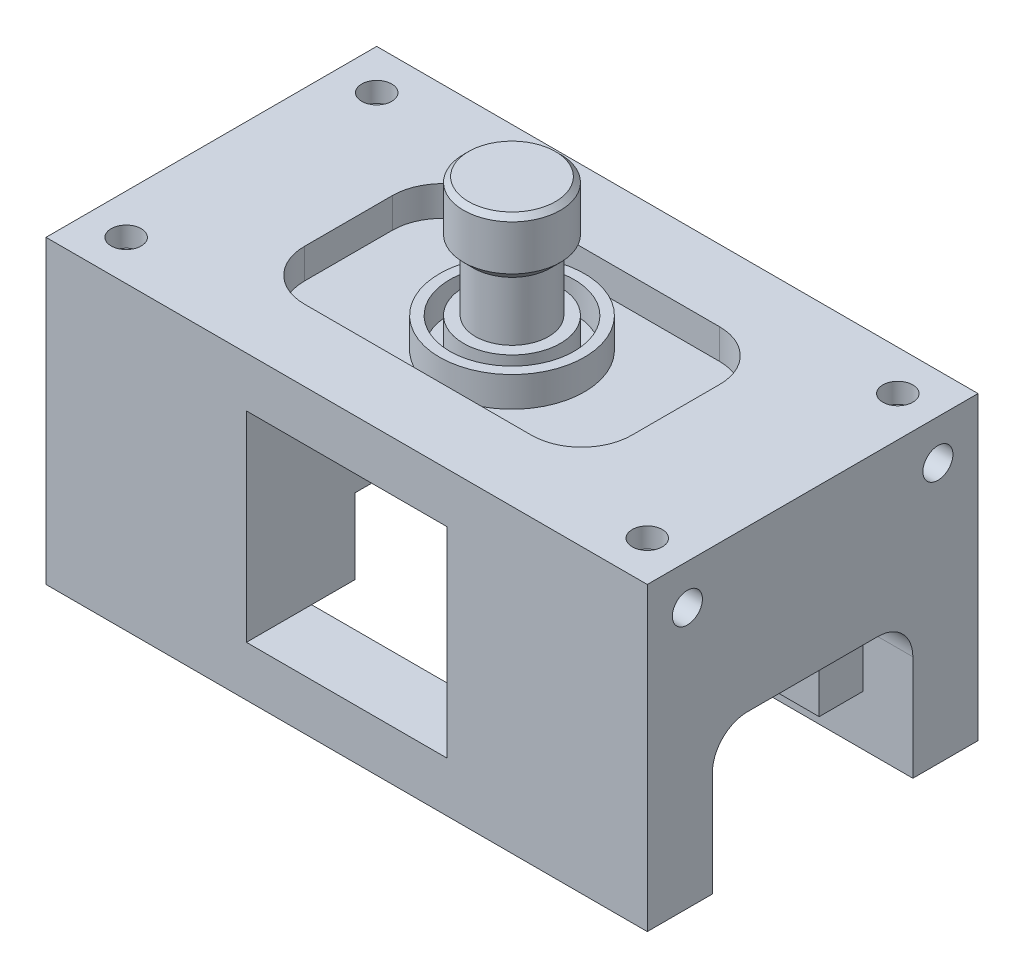
from build123d import *

# Parameters (mm, degrees)
SKETCH1_W           = 120
SKETCH1_H           = 66
BOSS_EXTRUDE1_DEPTH = 60
SKETCH3_W           = 40
SKETCH3_H           = 20
CUT_EXTRUDE1_DEPTH  = 120
SKETCH4_W           = 40
SKETCH4_H           = 40
CUT_EXTRUDE2_DEPTH  = 120
SKETCH5_W           = 22.599154532
SKETCH5_H           = 30
CUT_EXTRUDE3_DEPTH  = 120
SKETCH6_R           = 3
CUT_EXTRUDE4_DEPTH  = 120
SKETCH7_W           = 40
SKETCH7_H           = 18
CUT_EXTRUDE5_DEPTH  = 10
SKETCH8_W           = 40
SKETCH8_H           = 18
CUT_EXTRUDE6_DEPTH  = 10
SKETCH9_W           = 65.307661508
SKETCH9_H           = 37.522692198
CUT_EXTRUDE7_DEPTH  = 6
FILLET1_R           = 10
SKETCH10_R          = 3
CUT_EXTRUDE8_DEPTH  = 4
FILLET2_R           = 7
SKETCH11_R          = 14.45708456
SKETCH11_R_2        = 12.407691548
BOSS_EXTRUDE2_DEPTH = 6
SKETCH12_R          = 9.667792976
BOSS_EXTRUDE3_DEPTH = 6
SKETCH13_R          = 7.310717913
BOSS_EXTRUDE4_DEPTH = 12
SKETCH14_R          = 9.667792976
BOSS_EXTRUDE5_DEPTH = 12
CHAMFER1_SIZE       = 2
CHAMFER2_SIZE       = 1


with BuildPart() as part:
    # Sketch1 → Boss-Extrude1 (new body)
    with BuildSketch(Plane(origin=(0, 0, 0), x_dir=(1, 0, 0), z_dir=(0, 1, 0))):
        Rectangle(SKETCH1_W, SKETCH1_H)
    extrude(amount=BOSS_EXTRUDE1_DEPTH)

    # Sketch3 → Cut-Extrude1 (cut)
    with BuildSketch(Plane(origin=(60, 0, 0), x_dir=(0, 0, -1), z_dir=(1, 0, 0))):
        Rectangle(SKETCH3_W, SKETCH3_H)
    extrude(amount=-CUT_EXTRUDE1_DEPTH, mode=Mode.SUBTRACT)

    # Sketch4 → Cut-Extrude2 (cut)
    with BuildSketch(Plane.XY.offset(33)):
        with Locations((0, 30)):
            Rectangle(SKETCH4_W, SKETCH4_H)
    extrude(amount=-CUT_EXTRUDE2_DEPTH, mode=Mode.SUBTRACT)

    # Sketch5 → Cut-Extrude3 (cut)
    with BuildSketch(Plane(origin=(60, 0, 0), x_dir=(0, 0, -1), z_dir=(1, 0, 0))):
        with Locations((0, 10)):
            Rectangle(SKETCH5_W, SKETCH5_H)
    extrude(amount=-CUT_EXTRUDE3_DEPTH, mode=Mode.SUBTRACT)

    # Sketch6 → Cut-Extrude4 (cut)
    with BuildSketch(Plane(origin=(60, 0, 0), x_dir=(0, 0, -1), z_dir=(1, 0, 0))):
        with Locations((-25, 52)):
            Circle(SKETCH6_R)
        with Locations((25, 52)):
            Circle(SKETCH6_R)
    extrude(amount=-CUT_EXTRUDE4_DEPTH, mode=Mode.SUBTRACT)

    # Sketch7 → Cut-Extrude5 (cut)
    with BuildSketch(Plane(origin=(60, 0, 0), x_dir=(0, 0, -1), z_dir=(1, 0, 0))):
        with Locations((0, 19)):
            Rectangle(SKETCH7_W, SKETCH7_H)
    extrude(amount=-CUT_EXTRUDE5_DEPTH, mode=Mode.SUBTRACT)

    # Sketch8 → Cut-Extrude6 (cut)
    with BuildSketch(Plane.ZY.offset(60)):
        with Locations((0, 19)):
            Rectangle(SKETCH8_W, SKETCH8_H)
    extrude(amount=-CUT_EXTRUDE6_DEPTH, mode=Mode.SUBTRACT)

    # Sketch9 → Cut-Extrude7 (cut)
    with BuildSketch(Plane(origin=(0, 60, 0), x_dir=(1, 0, 0), z_dir=(0, 1, 0))):
        Rectangle(SKETCH9_W, SKETCH9_H)
    extrude(amount=-CUT_EXTRUDE7_DEPTH, mode=Mode.SUBTRACT)

    # Fillet1
    fillet1_edges = [part.edges().sort_by_distance(p)[0] for p in [
        (32.653830754, 57, -18.761346099),
        (32.653830754, 57, 18.761346099),
        (-32.653830754, 57, 18.761346099),
        (-32.653830754, 57, -18.761346099),
    ]]
    fillet(fillet1_edges, radius=FILLET1_R)

    # Sketch10 → Cut-Extrude8 (cut)
    with BuildSketch(Plane(origin=(0, 60, 0), x_dir=(1, 0, 0), z_dir=(0, 1, 0))):
        with Locations(Location((-52, 25, 0), (0, 0, 270))):
            Circle(SKETCH10_R)
        with Locations(Location((52, 25, 0), (0, 0, 270))):
            Circle(SKETCH10_R)
        with Locations(Location((-52, -25, 0), (0, 0, 270))):
            Circle(SKETCH10_R)
        with Locations(Location((52, -25, 0), (0, 0, 270))):
            Circle(SKETCH10_R)
    extrude(amount=-CUT_EXTRUDE8_DEPTH, mode=Mode.SUBTRACT)

    # Fillet2
    fillet2_edges = [part.edges().sort_by_distance(p)[0] for p in [
        (55, 28, 20),
        (55, 28, -20),
        (-55, 28, -20),
        (-55, 28, 20),
    ]]
    fillet(fillet2_edges, radius=FILLET2_R)

    # Sketch11 → Boss-Extrude2 (add)
    with BuildSketch(Plane(origin=(0, 54, 0), x_dir=(1, 0, 0), z_dir=(0, 1, 0))):
        with Locations(Location((0, 0, 0), (0, 0, 270))):
            Circle(SKETCH11_R)
        with Locations(Location((0, 0, 0), (0, 0, 270))):
            Circle(SKETCH11_R_2, mode=Mode.SUBTRACT)
    extrude(amount=BOSS_EXTRUDE2_DEPTH)

    # Sketch12 → Boss-Extrude3 (add)
    with BuildSketch(Plane(origin=(0, 54, 0), x_dir=(1, 0, 0), z_dir=(0, 1, 0))):
        with Locations(Location((0, 0, 0), (0, 0, 270))):
            Circle(SKETCH12_R)
    extrude(amount=BOSS_EXTRUDE3_DEPTH)

    # Sketch13 → Boss-Extrude4 (add)
    with BuildSketch(Plane(origin=(0, 60, 0), x_dir=(1, 0, 0), z_dir=(0, 1, 0))):
        with Locations(Location((0, 0, 0), (0, 0, 270))):
            Circle(SKETCH13_R)
    extrude(amount=BOSS_EXTRUDE4_DEPTH)

    # Sketch14 → Boss-Extrude5 (add)
    with BuildSketch(Plane(origin=(0, 72, 0), x_dir=(1, 0, 0), z_dir=(0, 1, 0))):
        with Locations(Location((0, 0, 0), (0, 0, 270))):
            Circle(SKETCH14_R)
    extrude(amount=BOSS_EXTRUDE5_DEPTH)

    # Chamfer1
    chamfer1_edges = [part.edges().sort_by_distance(p)[0] for p in [
        (0, 72, -9.667792976),
    ]]
    chamfer(chamfer1_edges, length=CHAMFER1_SIZE)

    # Chamfer2
    chamfer2_edges = [part.edges().sort_by_distance(p)[0] for p in [
        (0, 84, -9.667792976),
    ]]
    chamfer(chamfer2_edges, length=CHAMFER2_SIZE)


solid = part.part
